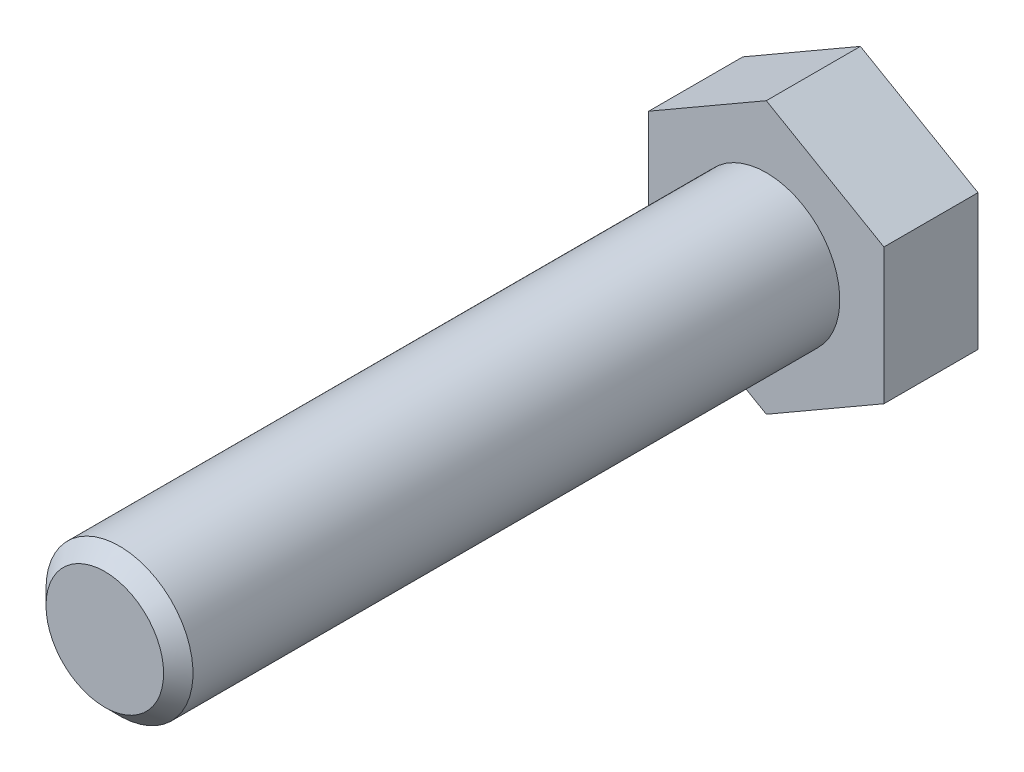
from build123d import *

# Parameters (mm, degrees)
BOSS_EXTRUDE1_DEPTH = 6.4
SKETCH3_R           = 5
BOSS_EXTRUDE2_DEPTH = 45
CHAMFER1_SIZE       = 1


with BuildPart() as part:
    # Sketch1 → Boss-Extrude1 (new body)
    with BuildSketch(Plane.XY):
        Polygon((8, 4.618802154), (0, 9.237604307), (-8, 4.618802154), (-8, -4.618802154), (0, -9.237604307), (8, -4.618802154), align=None)
    extrude(amount=BOSS_EXTRUDE1_DEPTH)

    # Sketch3 → Boss-Extrude2 (add)
    with BuildSketch(Plane.XY.offset(6.4)):
        with Locations(Location((0, 0, 0), (0, 0, 180))):
            Circle(SKETCH3_R)
    extrude(amount=BOSS_EXTRUDE2_DEPTH)

    # Chamfer1
    chamfer1_edges = [part.edges().sort_by_distance(p)[0] for p in [
        (5, 0, 51.4),
    ]]
    chamfer(chamfer1_edges, length=CHAMFER1_SIZE)


solid = part.part
